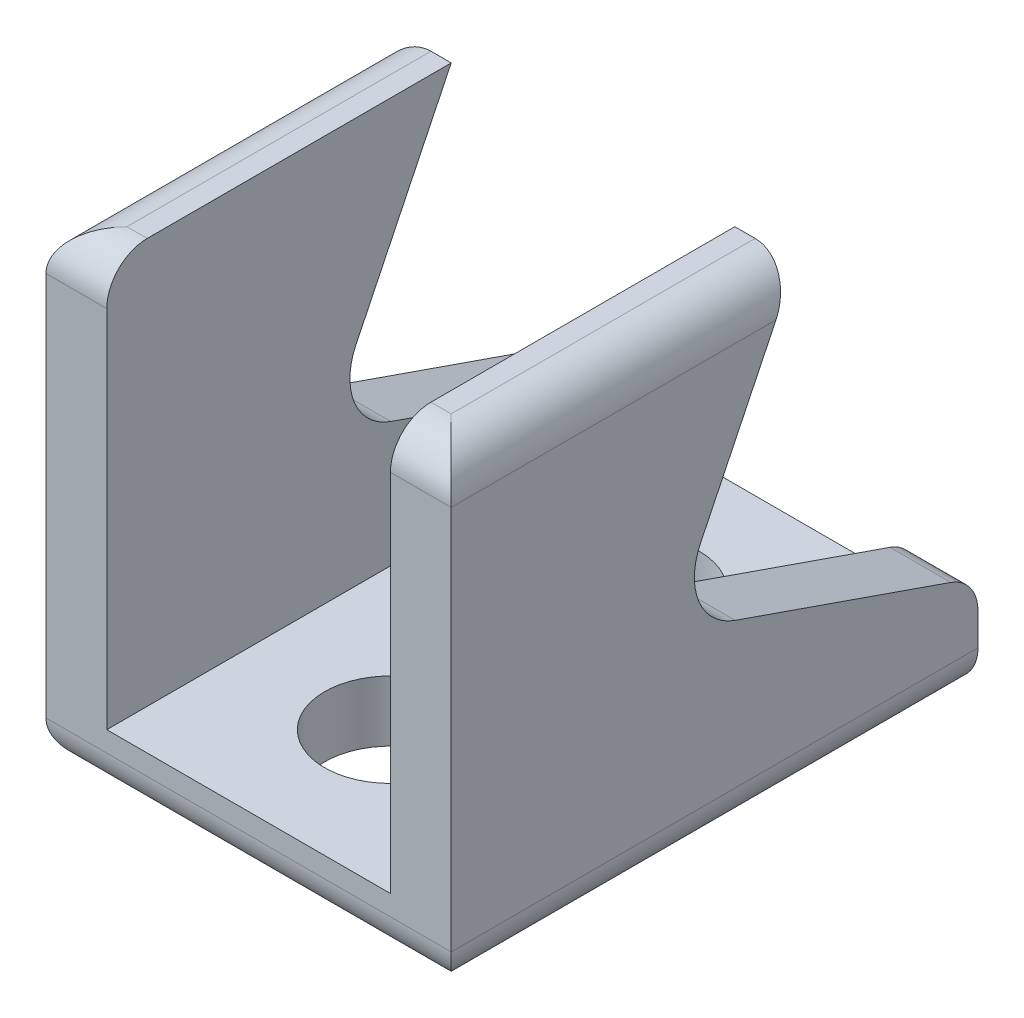
SolidWorks part; units mm, degrees
ref_plane "前视基准面" through (0, 0, 0) normal (0, 0, 1) x (1, 0, 0)
ref_plane "上视基准面" through (0, 0, 0) normal (0, 1, 0) x (1, 0, 0)
ref_plane "右视基准面" through (0, 0, 0) normal (1, 0, 0) x (0, 0, -1)
sketch "草图1" plane through (0, 0, 0) normal (1, 0, 0) x (0, 0, -1)
  line L0 (0, 23) -> (0, 0)
  line L1 (0, 0) -> (26, 0)
  line L2 (26, 0) -> (26, 5)
  line L3 (0, 23) -> (17, 23)
  line L4 (26, 5) -> (14.0149, 9.1663)
  line L5 (17, 23) -> (12.3006, 13.309)
  circle A0 centre (15, 12) radius 3
  dimension "D1" = 6
  dimension "D5" = 12
  dimension "D2" = 26
  dimension "D3" = 23
  dimension "D4" = 15
  dimension "D6" = 17
  dimension "D7" = 5
extrude "凸台-拉伸1" add sketch "草图1" along normal mid plane 20 contours A0 L5 L3 L0 L1 L2 L4
sketch "草图2" plane through (0, 0, 0) normal (1, 0, 0) x (0, 0, -1)
  line L0 (26, 0) -> (26, 5) construction
  line L1 (0, 23) -> (26, 23)
  line L2 (0, 23) -> (0, 3)
  line L3 (0, 3) -> (26, 3)
  line L4 (26, 23) -> (26, 3)
  line L5 (0, 0) -> (26, 0) construction
  dimension "D1" = 3
extrude "切除-拉伸1" cut sketch "草图2" against normal mid plane 14
sketch "草图3" plane through (0, 0, 0) normal (0, -1, 0) x (1, 0, 0)
  line L0 (10, 0) -> (-10, 0) construction
  line L1 (10, -26) -> (-10, -26) construction
  circle A0 centre (0, -7) radius 3.25
  circle A1 centre (0, -19) radius 3.25
  dimension "D1" = 6.5
  dimension "D2" = 6.5
  dimension "D3" = 7
  dimension "D4" = 7
extrude "切除-拉伸2" cut sketch "草图3" against normal up to next
fillet "圆角3" radius 2 9 edges at (8.5, 5, -26) (-8.5, 5, -26) (-10, 23, -8.5) (-10, 0, -13) (10, 0, -13) (10, 23, -8.5) (0, 0, 0) (-8.5, 23, 0) (8.5, 23, 0)
